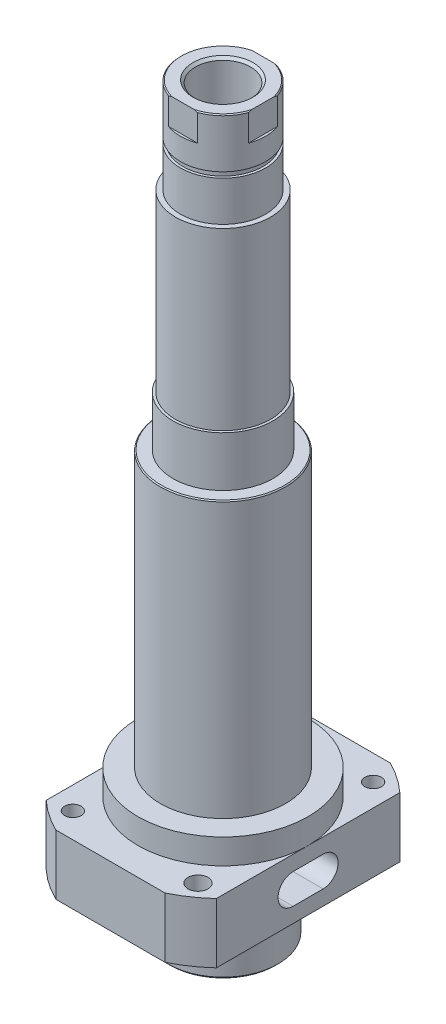
from build123d import *

# Parameters (mm, degrees)
SKETCH7_OUTSIDE_W   = 84.804
SKETCH7_OUTSIDE_H   = 84.804
SKETCH7_OUTSIDE_W_2 = 34
SKETCH7_OUTSIDE_H_2 = 45
CUT_EXTRUDE3_DEPTH  = 25
M4_TAPPED_HOLE2_D   = 3.3
SKETCH13_R          = 2
CUT_EXTRUDE6_DEPTH  = 25
SKETCH14_R          = 5.5
CUT_EXTRUDE7_DEPTH  = 151.66270275
CHAMFER1_SIZE       = 0.2
CHAMFER2_SIZE       = 0.5
SKETCH15_W          = 4.842021814
SKETCH15_H          = 7.203372967
CUT_EXTRUDE8_DEPTH  = 5
CUT_EXTRUDE9_DEPTH  = 154.513028763
SKETCH17_W          = 3.088959923
SKETCH17_H          = 8.04850145
SKETCH17_W_2        = 2.99848013
SKETCH17_H_2        = 8.967280155
CUT_EXTRUDE10_DEPTH = 5


with BuildPart() as part:
    # Sketch1 → Revolve1 (revolve)
    with BuildSketch(Plane.XY, mode=Mode.PRIVATE) as revolve1_sk:
        Polygon((0, 0), (11, 0), (11, 12), (25, 12), (25, 24), (17, 24), (17, 29), (12.5, 29), (12.5, 84), (10, 84), (10, 94), (9.5, 94), (9.5, 129), (8.5, 129), (8.5, 137), (8, 137), (8, 138.1), (8.5, 138.1), (8.5, 148), (0, 148), align=None)
    revolve(revolve1_sk.sketch.rotate(Axis((0, 148, 0), (0, -1, 0)), 90), axis=Axis((0, 148, 0), (0, -1, 0)))

    # Sketch7 outside → Cut-Extrude3 (cut)
    with BuildSketch(Plane(origin=(0, 24, 0), x_dir=(1, 0, 0), z_dir=(0, 1, 0))):
        Rectangle(SKETCH7_OUTSIDE_W, SKETCH7_OUTSIDE_H)
        Rectangle(SKETCH7_OUTSIDE_W_2, SKETCH7_OUTSIDE_H_2, mode=Mode.SUBTRACT)
    extrude(amount=-CUT_EXTRUDE3_DEPTH, mode=Mode.SUBTRACT)

    # M4 Tapped Hole2 (through all)
    with Locations(Plane(origin=(0, 12, 0), x_dir=(-1, 0, 0), z_dir=(0, -1, 0))):
        with Locations((-12.5, 17.5), (12.5, -17.5)):
            Hole(M4_TAPPED_HOLE2_D / 2)

    # Sketch13 → Cut-Extrude6 (cut)
    with BuildSketch(Plane.XZ.offset(-12)):
        with Locations(Location((12.5, 17.5, 0), (0, 0, 270))):
            Circle(SKETCH13_R)
        with Locations(Location((-12.5, -17.5, 0), (0, 0, 270))):
            Circle(SKETCH13_R)
    extrude(amount=-CUT_EXTRUDE6_DEPTH, mode=Mode.SUBTRACT)

    # Sketch14 → Cut-Extrude7 (cut, through all)
    with BuildSketch(Plane.XZ):
        Circle(SKETCH14_R)
    extrude(amount=-CUT_EXTRUDE7_DEPTH, mode=Mode.SUBTRACT)

    # Chamfer1
    chamfer1_edges = [part.edges().sort_by_distance(p)[0] for p in [
        (0, 148, -8.5),
        (0, 84, -12.5),
    ]]
    chamfer(chamfer1_edges, length=CHAMFER1_SIZE)

    # Chamfer2
    chamfer2_edges = [part.edges().sort_by_distance(p)[0] for p in [
        (-5.5, 148, 0),
        (-5.5, 0, 0),
        (0, 0, -11),
    ]]
    chamfer(chamfer2_edges, length=CHAMFER2_SIZE)

    # Sketch15 → Cut-Extrude8 (cut, symmetric)
    with BuildSketch(Plane.XY):
        with Locations((10.421010907, 146.101686484)):
            Rectangle(SKETCH15_W, SKETCH15_H)
    extrude(amount=CUT_EXTRUDE8_DEPTH, both=True, mode=Mode.SUBTRACT)

    # Sketch16 → Cut-Extrude9 (cut, through all)
    with BuildSketch(Plane.ZY.offset(17)):
        with BuildLine():
            Line((-3, 21), (3, 21))
            ThreePointArc((3, 21), (6, 18), (3, 15))
            Line((3, 15), (-3, 15))
            ThreePointArc((-3, 15), (-6, 18), (-3, 21))
        make_face()
    extrude(amount=-CUT_EXTRUDE9_DEPTH, mode=Mode.SUBTRACT)

    # Sketch17 → Cut-Extrude10 (cut, symmetric)
    with BuildSketch(Plane(origin=(0, 0, 0), x_dir=(0, 0, -1), z_dir=(1, 0, 0))):
        with Locations((9.544479962, 146.524250725)):
            Rectangle(SKETCH17_W, SKETCH17_H)
        with Locations((-9.499240065, 146.983640078)):
            Rectangle(SKETCH17_W_2, SKETCH17_H_2)
    extrude(amount=CUT_EXTRUDE10_DEPTH, both=True, mode=Mode.SUBTRACT)


solid = part.part
